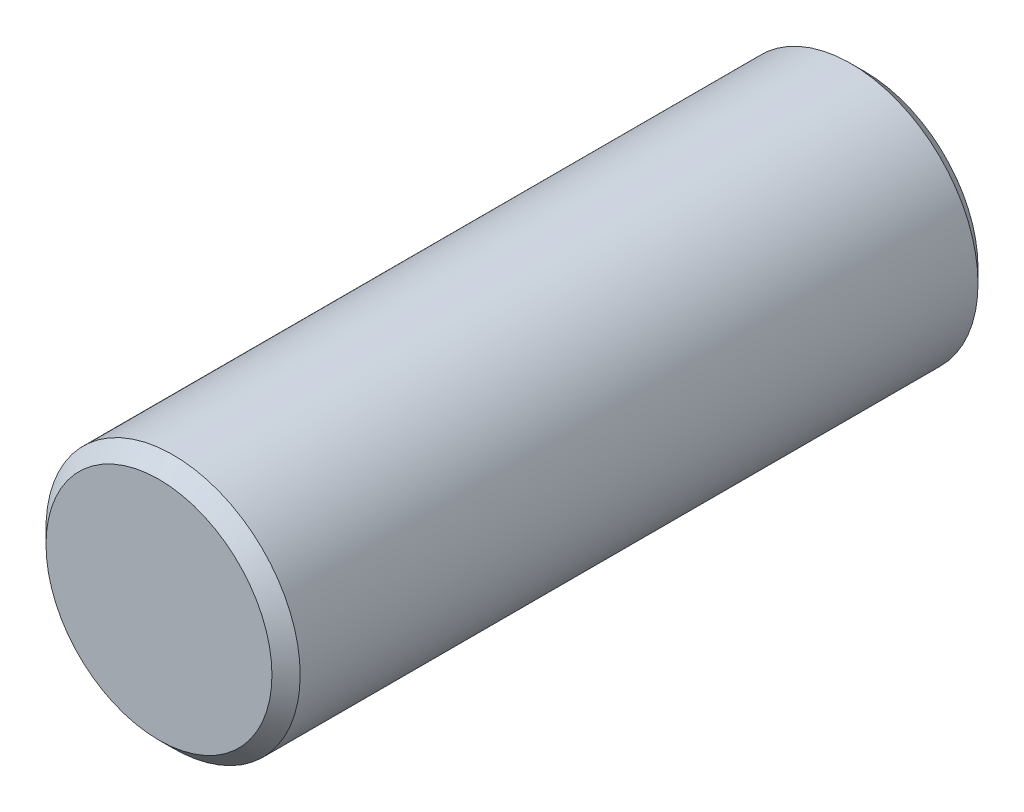
SolidWorks part; units mm, degrees
material "45"
ref_plane "Front Plane" through (0, 0, 0) normal (0, 0, 1) x (1, 0, 0)
ref_plane "Top Plane" through (0, 0, 0) normal (0, 1, 0) x (1, 0, 0)
ref_plane "Right Plane" through (0, 0, 0) normal (1, 0, 0) x (0, 0, -1)
sketch "Sketch1" plane through (0, 0, 0) normal (0, 0, 1) x (1, 0, 0)
  circle A0 centre (0, 0) radius 9
  dimension "D1" = 18
extrude "Boss-Extrude1" add sketch "Sketch1" along normal blind 50
chamfer "Chamfer1" distance 1 angle 45 2 edges at (9, 0, 0) (9, 0, 50)
sketch "Sketch2" plane through (0, 0, 0) normal (0, 0, -1) x (-1, 0, 0)
  line L0 (0, 0) -> (-14.823, 0) construction
